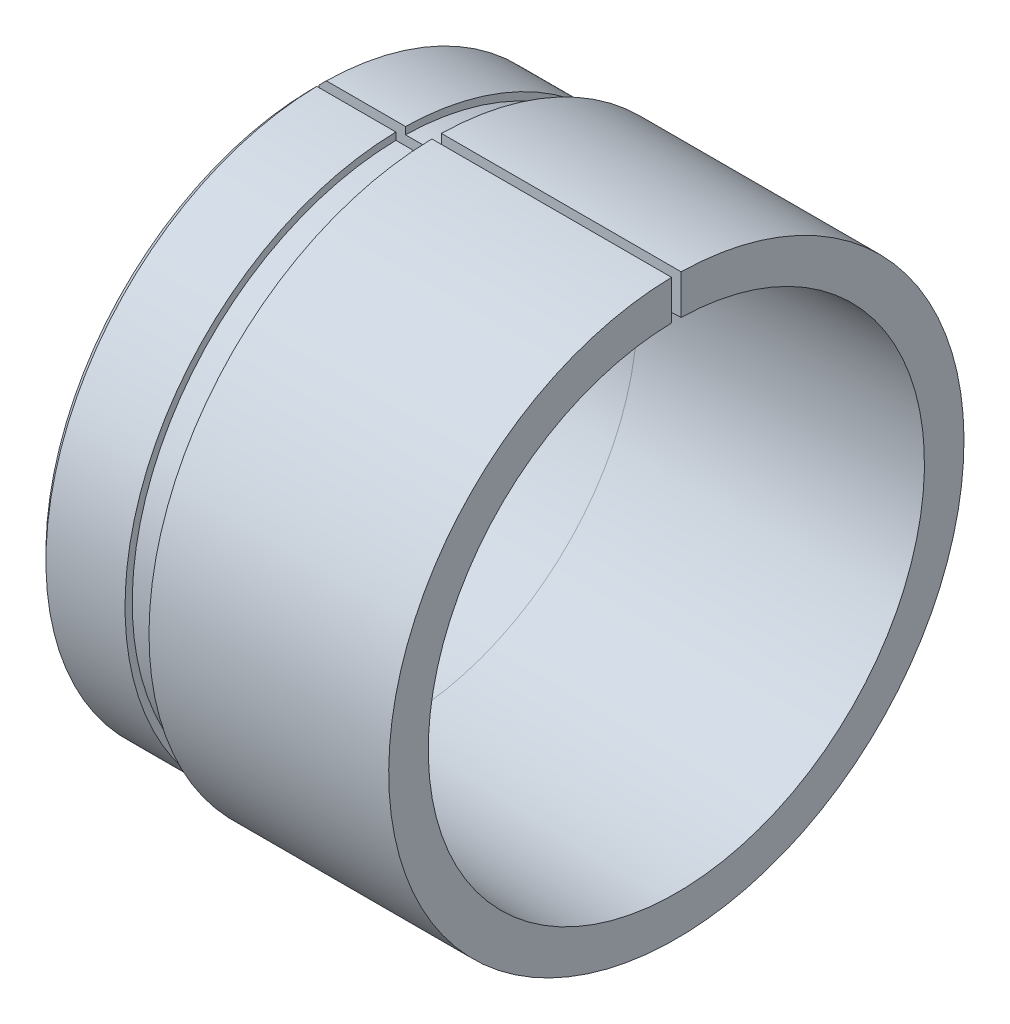
from build123d import *

# Parameters (mm, degrees)
CHAMFER1_SIZE      = 3
SKETCH2_W          = 4
SKETCH2_H          = 70.381112312
CUT_EXTRUDE2_DEPTH = 228.158534949


with BuildPart() as part:
    # Sketch1 → Revolve1 (revolve)
    with BuildSketch(Plane.XY, mode=Mode.PRIVATE) as revolve1_sk:
        Polygon((0, 115), (36, 115), (36, 112), (51, 112), (51, 120), (151, 120), (151, 103.5), (36, 98.7), (0, 98.7), align=None)
    revolve(revolve1_sk.sketch.rotate(Axis((0, 0, 0), (1, 0, 0)), 90), axis=Axis((0, 0, 0), (1, 0, 0)))

    # Chamfer1
    chamfer1_edges = [part.edges().sort_by_distance(p)[0] for p in [
        (0, 0, -115),
    ]]
    chamfer(chamfer1_edges, length=CHAMFER1_SIZE)

    # Sketch2 → Cut-Extrude2 (cut, through all)
    with BuildSketch(Plane(origin=(0, 0, 0), x_dir=(0, 0, -1), z_dir=(1, 0, 0))):
        with Locations((0, 103.5)):
            Rectangle(SKETCH2_W, SKETCH2_H)
    extrude(amount=CUT_EXTRUDE2_DEPTH, mode=Mode.SUBTRACT)


solid = part.part
